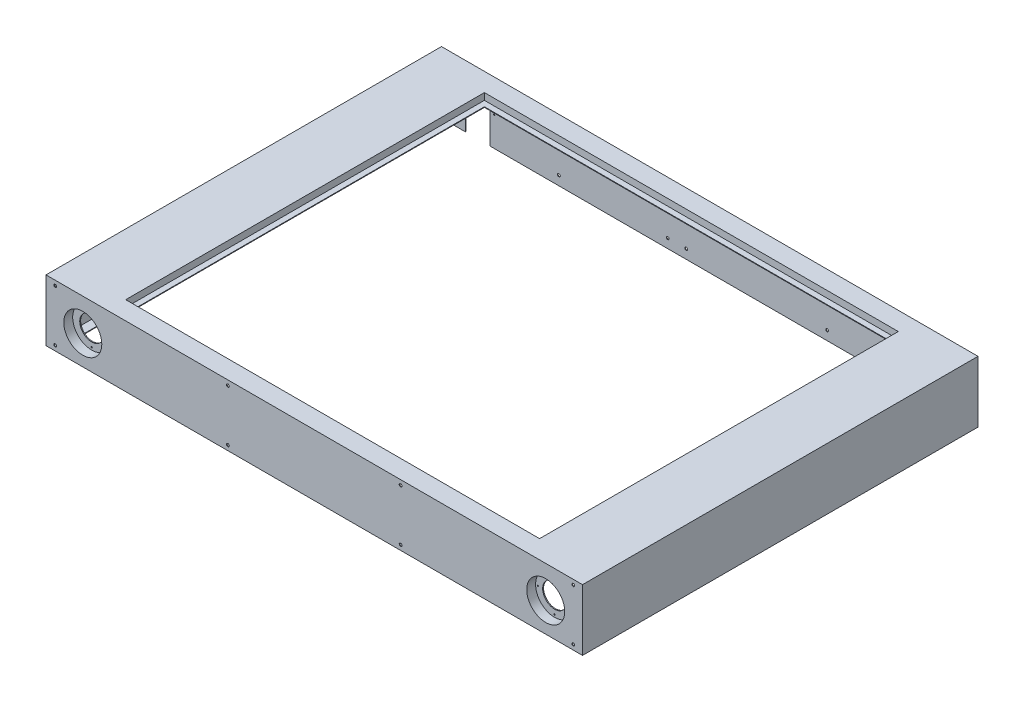
from build123d import *

# Parameters (mm, degrees)
SKETCH_1_W                  = 1750
SKETCH_1_H                  = 1290
EXTRUDE_1_DEPTH             = 2
SKETCH_2_W                  = 1350
SKETCH_2_H                  = 1170
CUT_EXTRUDE_1_DEPTH         = 2
SKETCH_3_W                  = 1290
SKETCH_3_H                  = 200
EXTRUDE_2_DEPTH             = 2
SKETCH_4_W                  = 1750
SKETCH_4_H                  = 200
EXTRUDE_3_DEPTH             = 2
SKETCH_5_W                  = 1750
SKETCH_5_H                  = 200
EXTRUDE_4_DEPTH             = 2
SKETCH_6_W                  = 1290
SKETCH_6_H                  = 200
EXTRUDE_5_DEPTH             = 2
SKETCH_7_W                  = 1350
SKETCH_7_H                  = 1170
EXTRUDE_6_DEPTH             = 24
SKETCH_8_W                  = 1354
SKETCH_8_H                  = 1174
SKETCH_8_W_2                = 1314
SKETCH_8_H_2                = 1134
EXTRUDE_7_DEPTH             = 2
EXTRUDE_8_DEPTH             = 2
CUT_EXTRUDE_2_DEPTH         = 2
SKETCH_11_R                 = 4.5
CUT_EXTRUDE_3_DEPTH         = 10
SKETCH_12_R                 = 4.5
CUT_EXTRUDE_4_DEPTH         = 10
SKETCH_13_R                 = 4.5
CUT_EXTRUDE_5_DEPTH         = 10
SKETCH_14_R                 = 4.5
CUT_EXTRUDE_6_DEPTH         = 8
SKETCH_16_R                 = 62
CUT_EXTRUDE_7_DEPTH         = 10
SKETCH_17_R                 = 64
SKETCH_17_R_2               = 62
EXTRUDE_9_DEPTH             = 27
SKETCH_22_R                 = 64
SKETCH_22_R_2               = 39
EXTRUDE_11_DEPTH            = 3
SKETCH_23_W                 = 2.1
SKETCH_23_H                 = 1261
HOLE_WIZARD_M5_1_AT_2_COUNT = 2
HOLE_WIZARD_M5_1_AT_2_PITCH = 54
HOLE_WIZARD_M5_1_AT_3_COUNT = 2
HOLE_WIZARD_M5_1_AT_3_PITCH = 104.319989239
HOLE_WIZARD_M5_1_AT_4_COUNT = 2
HOLE_WIZARD_M5_1_AT_4_PITCH = 123.845307359
MIRROR_3_COPY_1_SKETCH_W    = 2.1
MIRROR_3_COPY_1_SKETCH_H    = 1261
MIRROR_3_COPY_2_SKETCH_W    = 2.1
MIRROR_3_COPY_2_SKETCH_H    = 1261
MIRROR_3_COPY_3_SKETCH_W    = 2.1
MIRROR_3_COPY_3_SKETCH_H    = 1261


with BuildPart() as part:
    # 草图1 → 凸台-拉伸1 (new body)
    with BuildSketch(Plane(origin=(0, 0, 0), x_dir=(1, 0, 0), z_dir=(0, 1, 0))):
        Rectangle(SKETCH_1_W, SKETCH_1_H)
    extrude(amount=-EXTRUDE_1_DEPTH)

    # 草图2 → 切除-拉伸1 (cut)
    with BuildSketch(Plane(origin=(0, 0, 0), x_dir=(-1, 0, 0), z_dir=(0, 1, 0))):
        Rectangle(SKETCH_2_W, SKETCH_2_H)
    extrude(amount=-CUT_EXTRUDE_1_DEPTH, mode=Mode.SUBTRACT)

    # 草图3 → 凸台-拉伸2 (add)
    with BuildSketch(Plane(origin=(875, 0, 0), x_dir=(0, 0, -1), z_dir=(1, 0, 0))):
        with Locations((0, -100)):
            Rectangle(SKETCH_3_W, SKETCH_3_H)
    extrude(amount=-EXTRUDE_2_DEPTH)

    # 草图4 → 凸台-拉伸3 (add)
    with BuildSketch(Plane(origin=(0, 0, -645), x_dir=(-1, 0, 0), z_dir=(0, 0, -1))):
        with Locations((0, -100)):
            Rectangle(SKETCH_4_W, SKETCH_4_H)
    extrude(amount=-EXTRUDE_3_DEPTH)

    # 草图5 → 凸台-拉伸4 (add)
    with BuildSketch(Plane.XY.offset(645)):
        with Locations((0, -100)):
            Rectangle(SKETCH_5_W, SKETCH_5_H)
    extrude(amount=-EXTRUDE_4_DEPTH)

    # 草图6 → 凸台-拉伸5 (add)
    with BuildSketch(Plane.ZY.offset(875)):
        with Locations((0, -100)):
            Rectangle(SKETCH_6_W, SKETCH_6_H)
    extrude(amount=-EXTRUDE_5_DEPTH)

    # 草图7 → 凸台-拉伸6 (add)
    with BuildSketch(Plane(origin=(0, 0, 0), x_dir=(1, 0, 0), z_dir=(0, 1, 0))):
        Polygon((-677, 0), (-677, 587), (5, 587), (677, 587), (677, 0), (677, -587), (5, -587), (-677, -587), align=None)
        Rectangle(SKETCH_7_W, SKETCH_7_H, mode=Mode.SUBTRACT)
    extrude(amount=-EXTRUDE_6_DEPTH)

    # 草图8 → 凸台-拉伸7 (add)
    with BuildSketch(Plane.XZ.offset(24)):
        Rectangle(SKETCH_8_W, SKETCH_8_H)
        Rectangle(SKETCH_8_W_2, SKETCH_8_H_2, mode=Mode.SUBTRACT)
    extrude(amount=-EXTRUDE_7_DEPTH)

    # 草图9 → 凸台-拉伸8 (add)
    with BuildSketch(Plane.XZ.offset(200)):
        Polygon((-875, 645), (875, 645), (875, -645), (845, -645), (845, 615), (-845, 615), (-845, -610), (-845, -645), (-875, -645), align=None)
    extrude(amount=-EXTRUDE_8_DEPTH)

    # 草图10 → 切除-拉伸2 (cut)
    with BuildSketch(Plane(origin=(0, 0, -645), x_dir=(-1, 0, 0), z_dir=(0, 0, -1))):
        with BuildLine():
            Line((-795, -200), (-795, -105))
            ThreePointArc((-795, -105), (-755, -65), (-715, -105))
            Line((-715, -105), (-715, -200))
            Line((-715, -200), (-795, -200))
        make_face()
        with BuildLine():
            Line((715, -200), (715, -105))
            ThreePointArc((715, -105), (755, -65), (795, -105))
            Line((795, -105), (795, -200))
            Line((795, -200), (715, -200))
        make_face()
    extrude(amount=-CUT_EXTRUDE_2_DEPTH, mode=Mode.SUBTRACT)

    # 草图11 → 切除-拉伸3 (cut)
    with BuildSketch(Plane.XY.offset(-643)):
        with Locations((845, -30)):
            Circle(SKETCH_11_R)
        with Locations((845, -170)):
            Circle(SKETCH_11_R)
        with Locations((385, -30)):
            Circle(SKETCH_11_R)
        with Locations((385, -170)):
            Circle(SKETCH_11_R)
        with Locations((-75, -30)):
            Circle(SKETCH_11_R)
        with Locations((-75, -170)):
            Circle(SKETCH_11_R)
    extrude(amount=-CUT_EXTRUDE_3_DEPTH, mode=Mode.SUBTRACT)

    # 草图12 → 切除-拉伸4 (cut)
    with BuildSketch(Plane(origin=(0, 0, -645), x_dir=(-1, 0, 0), z_dir=(0, 0, -1))):
        with Locations((845, -30)):
            Circle(SKETCH_12_R)
        with Locations((845, -170)):
            Circle(SKETCH_12_R)
        with Locations((490, -30)):
            Circle(SKETCH_12_R)
        with Locations((490, -170)):
            Circle(SKETCH_12_R)
        with Locations((135, -30)):
            Circle(SKETCH_12_R)
        with Locations((135, -170)):
            Circle(SKETCH_12_R)
    extrude(amount=-CUT_EXTRUDE_4_DEPTH, mode=Mode.SUBTRACT)

    # 草图13 → 切除-拉伸5 (cut)
    with BuildSketch(Plane.XZ.offset(200)):
        with Locations(Location((-859, 615, 0), (0, 0, 270))):
            Circle(SKETCH_13_R)
        with Locations(Location((-859, -615, 0), (0, 0, 270))):
            Circle(SKETCH_13_R)
        with Locations(Location((859, -615, 0), (0, 0, 90))):
            Circle(SKETCH_13_R)
        with Locations(Location((859, 615, 0), (0, 0, 90))):
            Circle(SKETCH_13_R)
        with Locations(Location((859, 320, 0), (0, 0, 270))):
            Circle(SKETCH_13_R)
        with Locations(Location((859, -150, 0), (0, 0, 270))):
            Circle(SKETCH_13_R)
        with Locations(Location((-859, 302, 0), (0, 0, 270))):
            Circle(SKETCH_13_R)
        with Locations(Location((-859, -156.5, 0), (0, 0, 270))):
            Circle(SKETCH_13_R)
        with Locations(Location((-859, 362, 0), (0, 0, 270))):
            Circle(SKETCH_13_R)
        with Locations(Location((859, 380, 0), (0, 0, 270))):
            Circle(SKETCH_13_R)
    extrude(amount=-CUT_EXTRUDE_5_DEPTH, mode=Mode.SUBTRACT)

    # 草图14 → 切除-拉伸6 (cut)
    with BuildSketch(Plane.XY.offset(645)):
        with Locations((-845, -16)):
            Circle(SKETCH_14_R)
        with Locations((-281.666666667, -16)):
            Circle(SKETCH_14_R)
        with Locations((281.666666667, -16)):
            Circle(SKETCH_14_R)
        with Locations((845, -16)):
            Circle(SKETCH_14_R)
        with Locations((-845, -184)):
            Circle(SKETCH_14_R)
        with Locations((-281.666666667, -184)):
            Circle(SKETCH_14_R)
        with Locations((281.666666667, -184)):
            Circle(SKETCH_14_R)
        with Locations((845, -184)):
            Circle(SKETCH_14_R)
    extrude(amount=-CUT_EXTRUDE_6_DEPTH, mode=Mode.SUBTRACT)

    # 草图16 → 切除-拉伸7 (cut)
    with BuildSketch(Plane.XY.offset(645)):
        with Locations((755, -105)):
            Circle(SKETCH_16_R)
        with Locations((-755, -105)):
            Circle(SKETCH_16_R)
    extrude(amount=-CUT_EXTRUDE_7_DEPTH, mode=Mode.SUBTRACT)

    # 草图17 → 凸台-拉伸9 (add)
    with BuildSketch(Plane(origin=(0, 0, 643), x_dir=(-1, 0, 0), z_dir=(0, 0, -1))):
        with Locations(Location((-755, -105, 0), (0, 0, 180))):
            Circle(SKETCH_17_R)
        with Locations(Location((-755, -105, 0), (0, 0, 180))):
            Circle(SKETCH_17_R_2, mode=Mode.SUBTRACT)
    extrude_9 = extrude(amount=EXTRUDE_9_DEPTH)

    # 草图22 → 凸台-拉伸11 (add)
    with BuildSketch(Plane(origin=(0, 0, 616), x_dir=(-1, 0, 0), z_dir=(0, 0, -1))):
        with Locations(Location((-755, -105, 0), (0, 0, 180))):
            Circle(SKETCH_22_R)
        with Locations((-755, -105)):
            Circle(SKETCH_22_R_2, mode=Mode.SUBTRACT)
    extrude_11 = extrude(amount=EXTRUDE_11_DEPTH)

    # 镜向2: 凸台-拉伸9, 凸台-拉伸11 across plane
    add(extrude_9.mirror(Plane.ZY))
    add(extrude_11.mirror(Plane.ZY))

    # 草图23 → M5 螺纹孔1 (revolve, cut)
    with BuildSketch(Plane(origin=(728, -58.234628196, 616), x_dir=(0, -1, 0), z_dir=(1, 0, 0))):
        with Locations((1.05, 630.5)):
            Rectangle(SKETCH_23_W, SKETCH_23_H)
    hole_wizard_m5_1 = revolve(axis=Axis((728, -58.234628196, 622.35), (0, 0, -1)), mode=Mode.SUBTRACT)

    # M5 螺纹孔1 at 2: M5 螺纹孔1 ×2
    with Locations(*[Vector(-0.5000000000000002, -0.8660254037844386, 0) * (i * HOLE_WIZARD_M5_1_AT_2_PITCH) for i in range(1, HOLE_WIZARD_M5_1_AT_2_COUNT)]):
        add(hole_wizard_m5_1, mode=Mode.SUBTRACT)

    # M5 螺纹孔1 at 3: M5 螺纹孔1 ×2
    with Locations(*[Vector(0.25881904510252085, -0.9659258262890683, 0) * (i * HOLE_WIZARD_M5_1_AT_3_PITCH) for i in range(1, HOLE_WIZARD_M5_1_AT_3_COUNT)]):
        add(hole_wizard_m5_1, mode=Mode.SUBTRACT)

    # M5 螺纹孔1 at 4: M5 螺纹孔1 ×2
    with Locations(*[Vector(0.5813704332876158, -0.8136389981428925, 0) * (i * HOLE_WIZARD_M5_1_AT_4_PITCH) for i in range(1, HOLE_WIZARD_M5_1_AT_4_COUNT)]):
        add(hole_wizard_m5_1, mode=Mode.SUBTRACT)

    # 镜向3: M5 螺纹孔1 across plane
    add(hole_wizard_m5_1.mirror(Plane.ZY), mode=Mode.SUBTRACT)

    # 镜向3 copy 1 sketch → 镜向3 copy 1 (revolve, cut)
    with BuildSketch(Plane(origin=(-701, -105, 616), x_dir=(0, -1, 0), z_dir=(-1, 0, 0))):
        with Locations((1.05, -630.5)):
            Rectangle(MIRROR_3_COPY_1_SKETCH_W, MIRROR_3_COPY_1_SKETCH_H)
    revolve(axis=Axis((-701, -105, 622.35), (0, 0, 1)), mode=Mode.SUBTRACT)

    # 镜向3 copy 2 sketch → 镜向3 copy 2 (revolve, cut)
    with BuildSketch(Plane(origin=(-755, -159, 616), x_dir=(0, -1, 0), z_dir=(-1, 0, 0))):
        with Locations((1.05, -630.5)):
            Rectangle(MIRROR_3_COPY_2_SKETCH_W, MIRROR_3_COPY_2_SKETCH_H)
    revolve(axis=Axis((-755, -159, 622.35), (0, 0, 1)), mode=Mode.SUBTRACT)

    # 镜向3 copy 3 sketch → 镜向3 copy 3 (revolve, cut)
    with BuildSketch(Plane(origin=(-800, -159, 616), x_dir=(0, -1, 0), z_dir=(-1, 0, 0))):
        with Locations((1.05, -630.5)):
            Rectangle(MIRROR_3_COPY_3_SKETCH_W, MIRROR_3_COPY_3_SKETCH_H)
    revolve(axis=Axis((-800, -159, 622.35), (0, 0, 1)), mode=Mode.SUBTRACT)


solid = part.part
